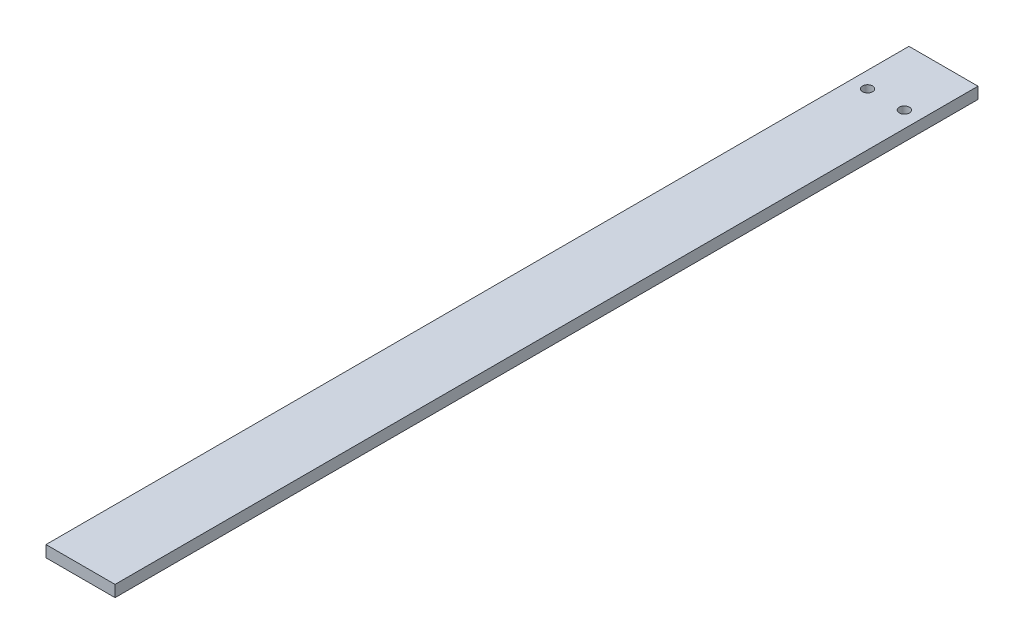
SolidWorks part; units mm, degrees
ref_plane "前视基准面" through (0, 0, 0) normal (0, 0, 1) x (1, 0, 0)
ref_plane "上视基准面" through (0, 0, 0) normal (0, 1, 0) x (1, 0, 0)
ref_plane "右视基准面" through (0, 0, 0) normal (1, 0, 0) x (0, 0, -1)
sketch "草图1" plane through (0, 0, 0) normal (0, 0, 1) x (1, 0, 0)
  line L1 (15, -2.5) -> (-15, -2.5)
  line L2 (15, -2.5) -> (15, 2.5)
  line L3 (15, 2.5) -> (-15, 2.5)
  line L4 (-15, -2.5) -> (-15, 2.5)
  line L5 (15, -2.5) -> (-15, 2.5) construction
  line L6 (15, 2.5) -> (-15, -2.5) construction
  point P0 (0, 0)
  dimension "D1" = 5
  dimension "D2" = 30
extrude "凸台-拉伸1" add sketch "草图1" along normal blind 15
sketch "草图2" plane through (0, 0, 0) normal (0, 0, -1) x (-1, 0, 0)
  line L0 (-15, -2.5) -> (-15, 2.5) construction
  line L1 (15, -5) -> (-15, -5)
  line L2 (15, -5) -> (15, 5)
  line L3 (15, 5) -> (-15, 5)
  line L4 (-15, -5) -> (-15, 5)
  line L5 (15, -5) -> (-15, 5) construction
  line L6 (15, 5) -> (-15, -5) construction
  point P0 (0, 0)
  dimension "D1" = 10
extrude "凸台-拉伸2" add sketch "草图2" along normal blind 172.5
mirror "镜向2" about plane through (0, 0, -172.5) normal (0, 0, -1) of bodies 107
sketch "草图3" plane through (0, 5, 0) normal (0, 1, 0) x (1, 0, 0)
  line L0 (0, 345) -> (0, 335) construction
  line L1 (-15, 345) -> (15, 345) construction
  line L2 (-8, 335) -> (8, 335) construction
  circle A6 centre (8, 335) radius 2.2
  circle A7 centre (-8, 335) radius 2.2
  dimension "D2" = 4.4
  dimension "D1" = 16
  dimension "D3" = 10
extrude "切除-拉伸1" cut sketch "草图3" against normal blind 10
sketch "草图4" plane through (0, 0, -345) normal (0, 0, -1) x (-1, 0, 0)
  line L4 (-15, 2.5) -> (15, 2.5)
  line L5 (15, 2.5) -> (15, 5)
  line L6 (15, 5) -> (-15, 5)
  line L7 (-15, 5) -> (-15, 2.5)
  line L8 (-15, 2.5) -> (15, 2.5)
  line L9 (15, 2.5) -> (15, 5)
  line L10 (15, 5) -> (-15, 5)
  line L11 (-15, 5) -> (-15, 2.5)
  line L12 (15, -2.5) -> (-15, -2.5)
  line L13 (-15, -2.5) -> (-15, -5)
  line L14 (-15, -5) -> (15, -5)
  line L15 (15, -5) -> (15, -2.5)
  line L16 (15, -2.5) -> (-15, -2.5)
  line L17 (-15, -2.5) -> (-15, -5)
  line L18 (-15, -5) -> (15, -5)
  line L19 (15, -5) -> (15, -2.5)
  dimension "D1" = 0
  dimension "D2" = 0
extrude "凸台-拉伸3" add sketch "草图4" along normal up to surface (15 mm away) up to face at (0, 0, -360)
sketch "草图5" plane through (0, 0, 0) normal (0, 0, 1) x (1, 0, 0)
  line L4 (-15, 2.5) -> (15, 2.5)
  line L5 (15, 2.5) -> (15, 5)
  line L6 (15, 5) -> (-15, 5)
  line L7 (-15, 5) -> (-15, 2.5)
  line L8 (-15, 2.5) -> (15, 2.5)
  line L9 (15, 2.5) -> (15, 5)
  line L10 (15, 5) -> (-15, 5)
  line L11 (-15, 5) -> (-15, 2.5)
  line L12 (15, -2.5) -> (-15, -2.5)
  line L13 (-15, -2.5) -> (-15, -5)
  line L14 (-15, -5) -> (15, -5)
  line L15 (15, -5) -> (15, -2.5)
  line L16 (15, -2.5) -> (-15, -2.5)
  line L17 (-15, -2.5) -> (-15, -5)
  line L18 (-15, -5) -> (15, -5)
  line L19 (15, -5) -> (15, -2.5)
  dimension "D1" = 0
  dimension "D2" = 0
extrude "凸台-拉伸4" add sketch "草图5" along normal up to surface (15 mm away) up to face at (0, 0, 15)
sketch "草图6" plane through (0, 5, 0) normal (0, 1, 0) x (1, 0, 0)
  line L4 (-15, 360) -> (-15, -15)
  line L5 (-15, -15) -> (15, -15)
  line L6 (15, -15) -> (15, 360)
  line L7 (15, 360) -> (-15, 360)
  line L8 (-15, 360) -> (-15, -15)
  line L9 (-15, -15) -> (15, -15)
  line L10 (15, -15) -> (15, 360)
  line L11 (15, 360) -> (-15, 360)
  dimension "D1" = 0
extrude "切除-拉伸2" cut sketch "草图6" against normal blind 5
